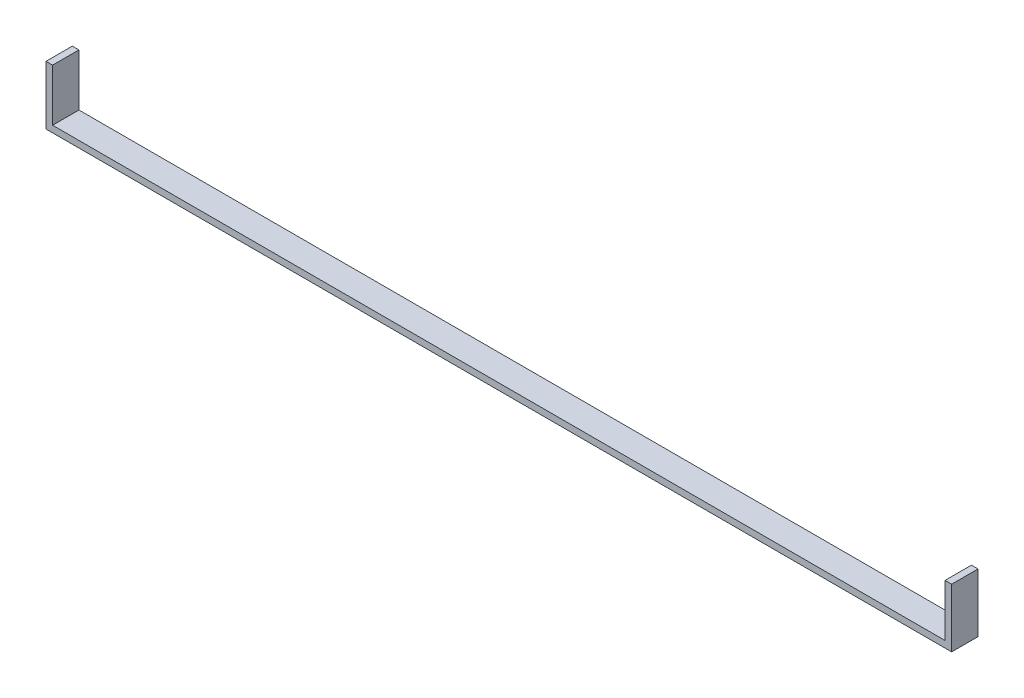
SolidWorks part; units mm, degrees
ref_plane "前视基准面" through (0, 0, 0) normal (0, 0, 1) x (1, 0, 0)
ref_plane "上视基准面" through (0, 0, 0) normal (0, 1, 0) x (1, 0, 0)
ref_plane "右视基准面" through (0, 0, 0) normal (1, 0, 0) x (0, 0, -1)
other "Configuration Table"
sketch "草图1" plane through (0, 0, 0) normal (0, 1, 0) x (1, 0, 0)
  line L1 (-677, 20) -> (677, 20)
  line L2 (-677, 20) -> (-677, -20)
  line L3 (-677, -20) -> (677, -20)
  line L4 (677, 20) -> (677, -20)
  line L5 (-677, 20) -> (677, -20) construction
  line L6 (-677, -20) -> (677, 20) construction
  point P0 (0, 0)
  dimension "D1" = 40
  dimension "D2" = 1354
extrude "凸台-拉伸1" add sketch "草图1" along normal blind 10
sketch "草图2" plane through (-677, 0, 0) normal (-1, 0, 0) x (0, 0, 1)
  line L0 (-20, 10) -> (20, 10) construction
  line L1 (-20, 0) -> (20, 0)
  line L2 (-20, 0) -> (-20, 89)
  line L3 (-20, 89) -> (20, 89)
  line L4 (20, 0) -> (20, 89)
  point P7 (20, 0)
  dimension "D1" = 79
extrude "凸台-拉伸2" add sketch "草图2" along normal blind 10
mirror "镜向1" about plane through (0, 0, 0) normal (1, 0, 0) of "凸台-拉伸2"
